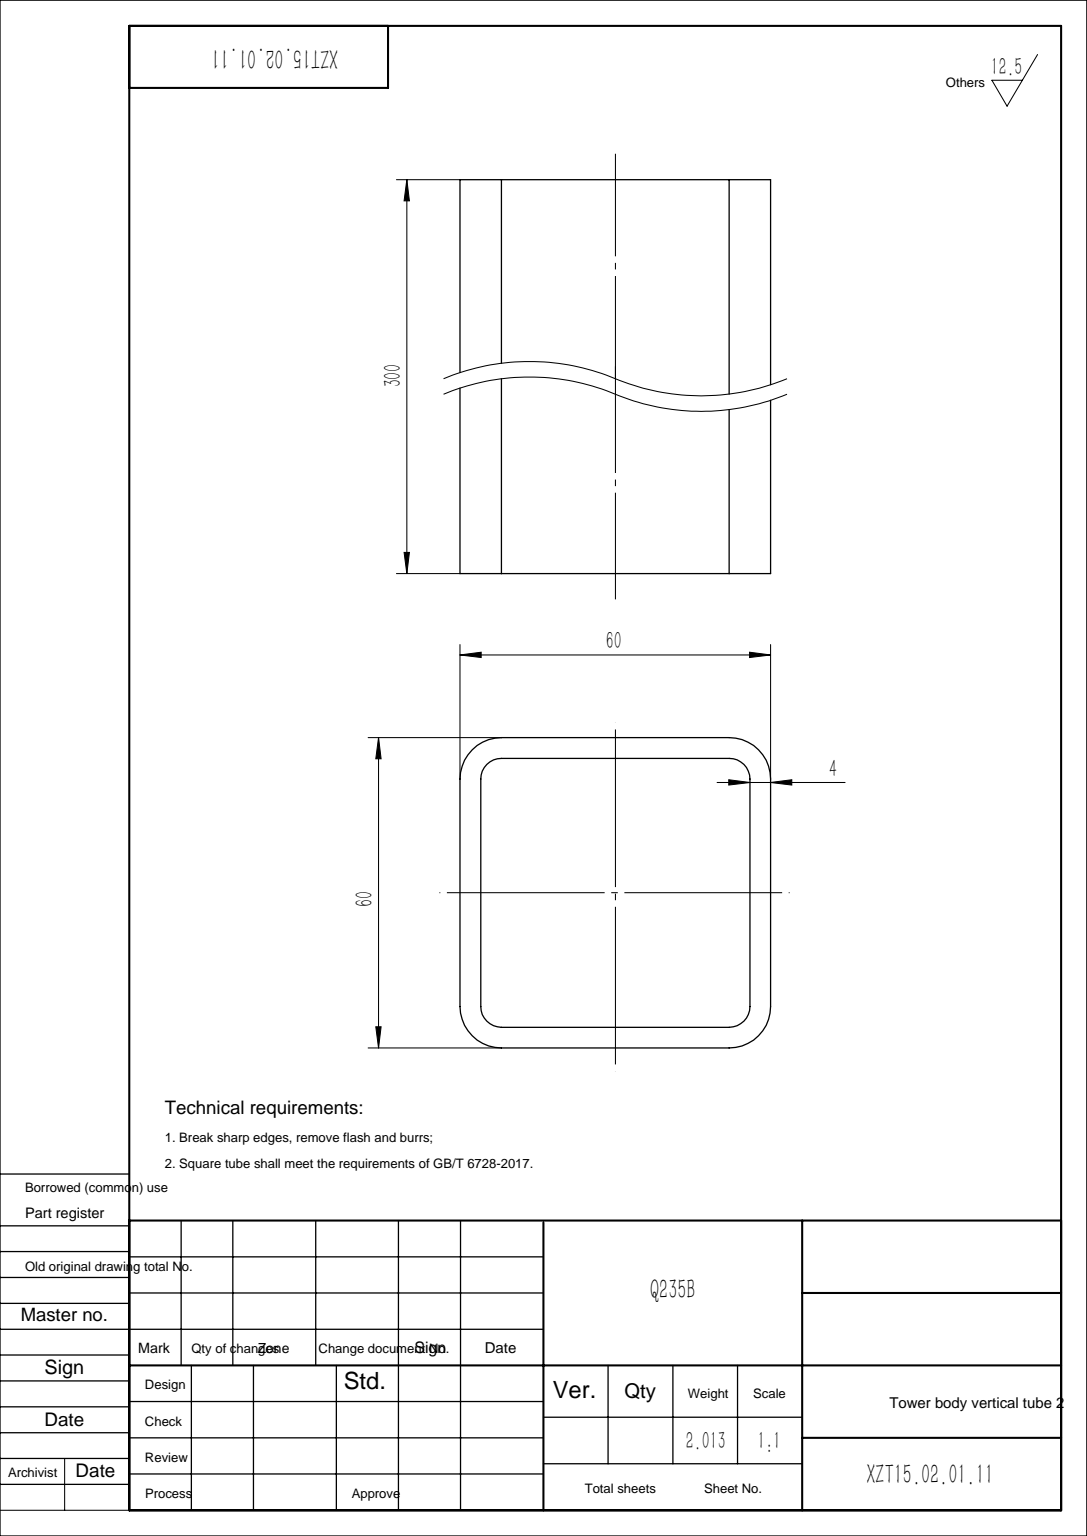
SolidWorks part; units mm, degrees
material "Q235B"
ref_plane "Front Plane" through (0, 0, 0) normal (0, 0, 1) x (1, 0, 0)
ref_plane "Top Plane" through (0, 0, 0) normal (0, 1, 0) x (1, 0, 0)
ref_plane "Right Plane" through (0, 0, 0) normal (1, 0, 0) x (0, 0, -1)
sketch "草图1" plane through (0, 0, 0) normal (0, 0, 1) x (1, 0, 0)
  line L0 (0, 0) -> (0, 300)
  dimension "D1" = 300
other "GB/T 6728-2002 square hollow section 60×60×4(1)"
ref_plane "Plane1" through (0, 0, 0) normal (0, 1, 0) x (-1, 0, 0)
sketch "Sketch1" plane through (0, 0, 0) normal (0, 1, 0) x (-1, 0, 0)
  line L0 (-22, -26) -> (22, -26)
  line L1 (-26, -22) -> (-26, 22)
  line L2 (22, 26) -> (-22, 26)
  line L3 (26, 22) -> (26, -22)
  line L4 (-22, -30) -> (22, -30)
  line L5 (-30, -22) -> (-30, 22)
  line L6 (22, 30) -> (-22, 30)
  line L7 (30, 22) -> (30, -22)
  arc A0 (30, 22) -> (22, 30) centre (22, 22) ccw
  arc A1 (22, -30) -> (30, -22) centre (22, -22) ccw
  arc A2 (-30, -22) -> (-22, -30) centre (-22, -22) ccw
  arc A3 (-22, 30) -> (-30, 22) centre (-22, 22) ccw
  arc A4 (-22, 26) -> (-26, 22) centre (-22, 22) ccw
  arc A5 (26, 22) -> (22, 26) centre (22, 22) ccw
  arc A6 (22, -26) -> (26, -22) centre (22, -22) ccw
  arc A7 (-26, -22) -> (-22, -26) centre (-22, -22) ccw
  point P0 (-30, 0)
  point P1 (30, 0)
  point P2 (0, 30)
  point P3 (0, -30)
  point P4 (0, 0)
  point P5 (-30, -30)
  point P6 (30, -30)
  point P7 (30, 30)
  point P8 (-30, 30)
  point P33 (0, 0)
  dimension "D1" = 8
  dimension "Thickness" = 4
  dimension "V_leg" = 60
